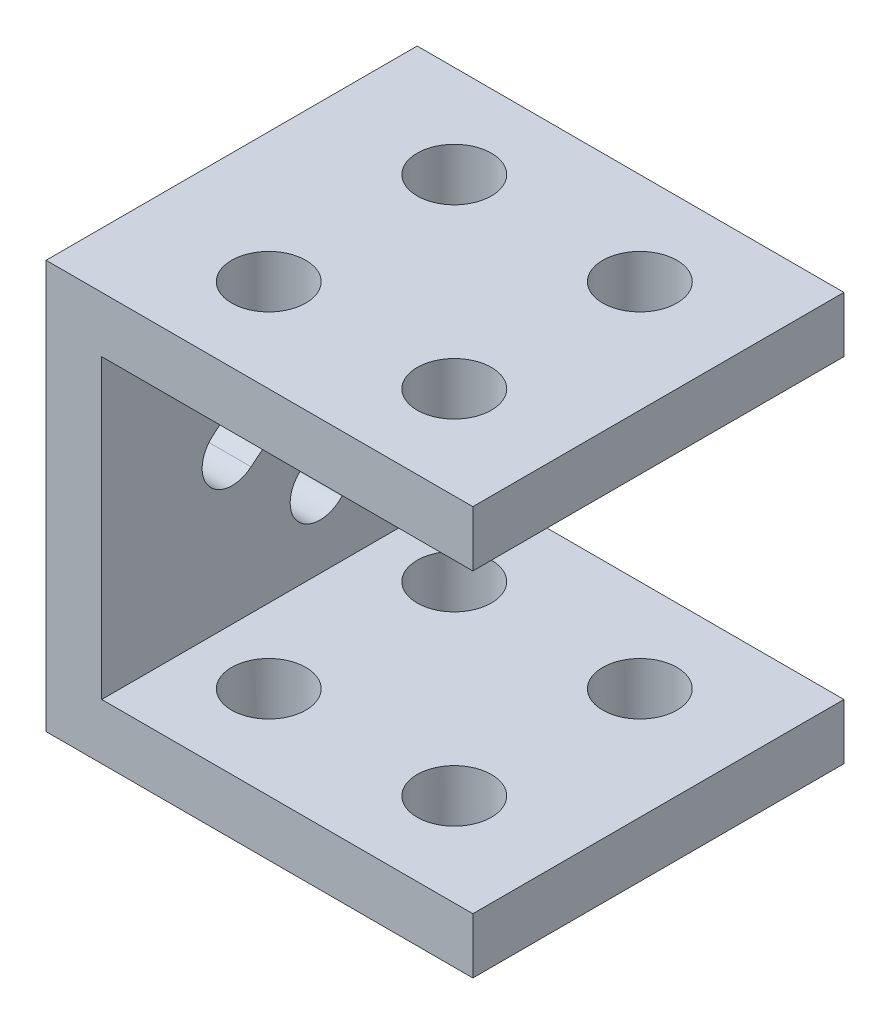
SolidWorks part; units mm, degrees
ref_plane "Front Plane" through (0, 0, 0) normal (0, 0, 1) x (1, 0, 0)
ref_plane "Top Plane" through (0, 0, 0) normal (0, 1, 0) x (1, 0, 0)
ref_plane "Right Plane" through (0, 0, 0) normal (1, 0, 0) x (0, 0, -1)
other "Configuration Table"
sketch "Sketch1" plane through (0, 0, 0) normal (0, 0, 1) x (1, 0, 0)
  line L0 (0, 0) -> (100, 0)
  line L1 (0, 0) -> (0, 80)
  line L2 (0, 80) -> (100, 80)
  line L3 (-15, -15) -> (100, -15)
  line L4 (-15, -15) -> (-15, 95)
  line L5 (-15, 95) -> (100, 95)
  line L6 (100, 95) -> (100, 80)
  line L7 (100, 0) -> (100, -15)
  dimension "D1" = 80
  dimension "D2" = 100
  dimension "D3" = 100
  dimension "D4" = 15
extrude "Boss-Extrude1" add sketch "Sketch1" along normal blind 100
sketch "Sketch2" plane through (0, 95, 0) normal (0, 1, 0) x (1, 0, 0)
  line L0 (100, -100) -> (-15, -100) construction
  line L1 (-15, -100) -> (-15, 0) construction
  line L2 (100, -100) -> (100, 0) construction
  circle A0 centre (20, -25) radius 10
  circle A1 centre (70, -25) radius 10
  circle A2 centre (20, -75) radius 10
  circle A3 centre (70, -75) radius 10
  dimension "D9" = 20
  dimension "D1" = 25
  dimension "D2" = 50
  dimension "D3" = 25
  dimension "D4" = 50
  dimension "D5" = 35
  dimension "D6" = 30
  dimension "D7" = 50
  dimension "D8" = 35
extrude "Cut-Extrude1" cut sketch "Sketch2" against normal blind 500
sketch "Sketch3" plane through (0, 0, 0) normal (1, 0, 0) x (0, 0, -1)
  line L0 (-64.8731, 40.4173) -> (-45.8574, 56.0039) construction
  line L3 (-69.9894, 46.659) -> (-50.9736, 62.2457)
  line L4 (-59.7569, 34.1755) -> (-40.7412, 49.7621)
  line L11 (-41.2031, 20.4904) -> (-23.9788, 39.5548) construction
  line L12 (-47.157, 25.8697) -> (-29.9328, 44.934)
  line L13 (-35.2491, 15.1112) -> (-18.0249, 34.1755)
  arc A2 (-69.9894, 46.659) -> (-59.7569, 34.1755) centre (-64.8731, 40.4173) ccw
  arc A3 (-40.7412, 49.7621) -> (-50.9736, 62.2457) centre (-45.8574, 56.0039) ccw
  arc A8 (-47.157, 25.8697) -> (-35.2491, 15.1112) centre (-41.2031, 20.4904) ccw
  arc A9 (-18.0249, 34.1755) -> (-29.9328, 44.934) centre (-23.9788, 39.5548) ccw
  point P2 (-55.3653, 48.2106)
  point P21 (-32.591, 30.0226)
extrude "Cut-Extrude2" cut sketch "Sketch3" against normal blind 500
